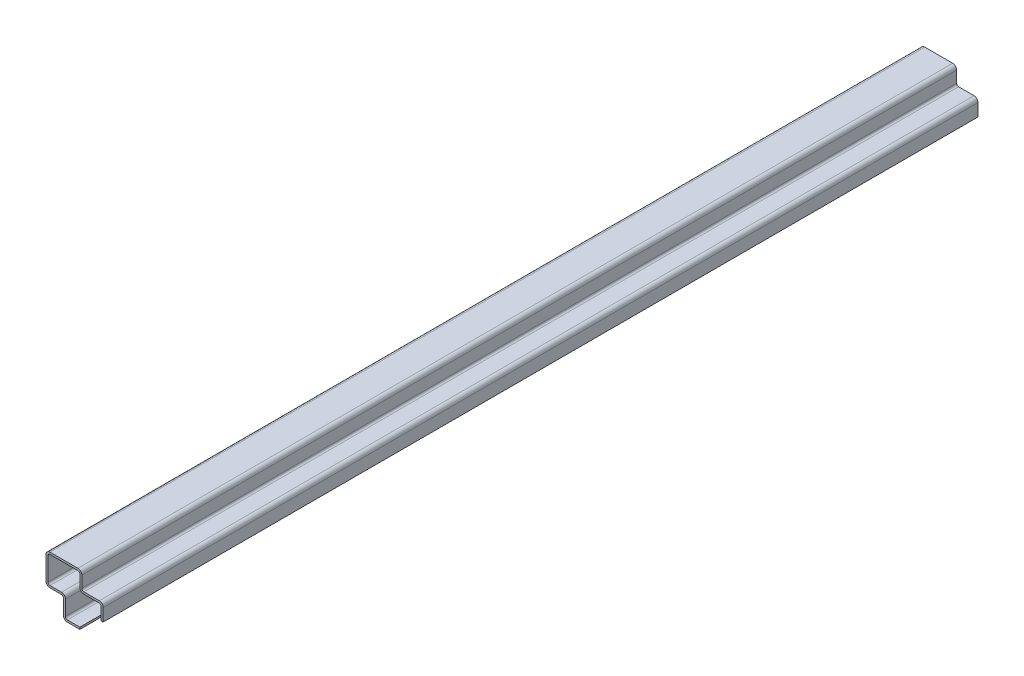
from build123d import *

# Parameters (mm, degrees)
BOSS_EXTRUDE1_DEPTH = 2660


with BuildPart() as part:
    # Sketch1 → Boss-Extrude1 (new body)
    with BuildSketch(Plane.XY):
        with BuildLine():
            Line((0, 0), (0, 38))
            ThreePointArc((0, 38), (-3.514718626, 46.485281374), (-12, 50))
            Line((-12, 50), (-59, 50))
            ThreePointArc((-59, 50), (-63.242640687, 51.757359313), (-65, 56))
            Line((-65, 56), (-65, 91))
            ThreePointArc((-65, 91), (-68.514718626, 99.485281374), (-77, 103))
            Line((-77, 103), (-162, 103))
            ThreePointArc((-162, 103), (-170.485281374, 99.485281374), (-174, 91))
            Line((-174, 91), (-174, 21))
            ThreePointArc((-174, 21), (-170.485281374, 12.514718626), (-162, 9))
            Line((-162, 9), (-127, 9))
            ThreePointArc((-127, 9), (-122.757359313, 7.242640687), (-121, 3))
            Line((-121, 3), (-121, -43))
            ThreePointArc((-121, -43), (-117.485281374, -51.485281374), (-109, -55))
            Line((-109, -55), (-71, -55))
            Line((-71, -55), (-71, -49))
            Line((-71, -49), (-109, -49))
            ThreePointArc((-109, -49), (-113.242640687, -47.242640687), (-115, -43))
            Line((-115, -43), (-115, 3))
            ThreePointArc((-115, 3), (-118.514718626, 11.485281374), (-127, 15))
            Line((-127, 15), (-162, 15))
            ThreePointArc((-162, 15), (-166.242640687, 16.757359313), (-168, 21))
            Line((-168, 21), (-168, 91))
            ThreePointArc((-168, 91), (-166.242640687, 95.242640687), (-162, 97))
            Line((-162, 97), (-77, 97))
            ThreePointArc((-77, 97), (-72.757359313, 95.242640687), (-71, 91))
            Line((-71, 91), (-71, 56))
            ThreePointArc((-71, 56), (-67.485281374, 47.514718626), (-59, 44))
            Line((-59, 44), (-12, 44))
            ThreePointArc((-12, 44), (-7.757359313, 42.242640687), (-6, 38))
            Line((-6, 38), (-6, 0))
            Line((-6, 0), (0, 0))
        make_face()
    extrude(amount=BOSS_EXTRUDE1_DEPTH)


solid = part.part
